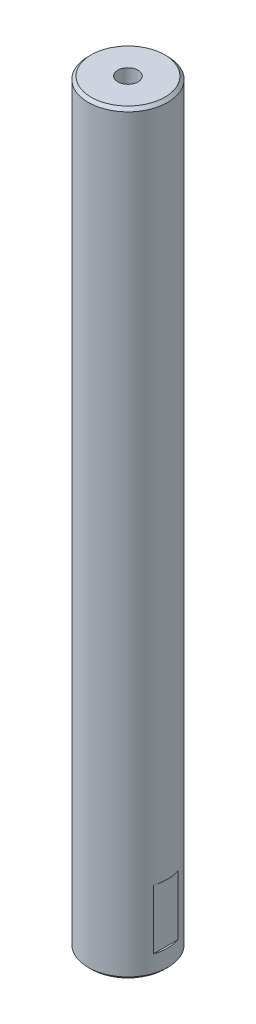
SolidWorks part; units mm, degrees
ref_plane "Front Plane" through (0, 0, 0) normal (0, 0, 1) x (1, 0, 0)
ref_plane "Top Plane" through (0, 0, 0) normal (0, 1, 0) x (1, 0, 0)
ref_plane "Right Plane" through (0, 0, 0) normal (1, 0, 0) x (0, 0, -1)
sketch "Sketch1" plane through (0, 0, 0) normal (0, 0, 1) x (1, 0, 0)
  line L1 (-108.7461, 325.3373) -> (-88.7461, 325.3373)
  line L2 (-108.7461, 325.3373) -> (-108.7461, -54.6627)
  line L3 (-108.7461, -54.6627) -> (-88.7461, -54.6627)
  line L4 (-88.7461, 325.3373) -> (-88.7461, -54.6627)
  line L5 (-108.7461, 325.3373) -> (-88.7461, -54.6627) construction
  line L6 (-108.7461, -54.6627) -> (-88.7461, 325.3373) construction
  point P0 (-98.7461, 135.3373)
  dimension "D1" = 380
  dimension "D2" = 20
revolve "Revolve1" add sketch "Sketch1" angle 360 about L4
sketch "Sketch2" plane through (0, 0, 0) normal (0, 0, 1) x (1, 0, 0)
  line L0 (-88.7461, 325.3373) -> (-88.7461, -54.6627) construction
  line L1 (-68.7461, 325.3373) -> (-108.7461, 325.3373) construction
  line L2 (-108.7461, -54.6627) -> (-68.7461, -54.6627) construction
  line L3 (-108.7461, 325.3373) -> (-108.7461, -54.6627) construction
  line L4 (-108.7461, -14.6627) -> (-107.7461, -14.6627)
  line L5 (-108.7461, -14.6627) -> (-108.7461, -44.6627)
  line L6 (-108.7461, -44.6627) -> (-107.7461, -44.6627)
  line L7 (-107.7461, -14.6627) -> (-107.7461, -44.6627)
  line L8 (-69.7461, -14.6627) -> (-69.7461, -44.6627)
  line L9 (-68.7461, -44.6627) -> (-69.7461, -44.6627)
  line L10 (-68.7461, -14.6627) -> (-68.7461, -44.6627)
  line L11 (-68.7461, -14.6627) -> (-69.7461, -14.6627)
  dimension "D1" = 30
  dimension "D2" = 340
  dimension "D3" = 1
extrude "Cut-Extrude1" cut sketch "Sketch2" against normal through all both and the other way through all
chamfer "Chamfer1" distance 1.5 angle 45 2 edges at (-88.7461, 325.3373, 20) (-88.7461, -54.6627, 20)
hole_wizard "M12 Tapped Hole1" positions "Sketch3" profile "Sketch4" tap size "M12" standard "GB"
sketch "Sketch3" plane through (0, 325.3373, 0) normal (0, 1, 0) x (1, 0, 0)
  point P0 (-88.7461, 0)
sketch "Sketch4" plane through (-88.7461, 325.3373, 0) normal (1, 0, 0) x (0, 0, 1)
  line L0 (0, 0) -> (0, 27.0644)
  line L1 (0, 27.0644) -> (5.1, 24)
  line L2 (5.1, 24) -> (5.1, 0)
  line L5 (5.1, 0) -> (0, 0)
  line L10 (0, 27.0644) -> (-5.1, 24) construction
  line L11 (0, -6.35) -> (0, 107.95) construction
  dimension "螺纹孔钻头直径" = 10.2
  dimension "螺纹孔钻头深度" = 24
  dimension "导头角度" = 118
cosmetic thread "Cosmetic thread 1"
